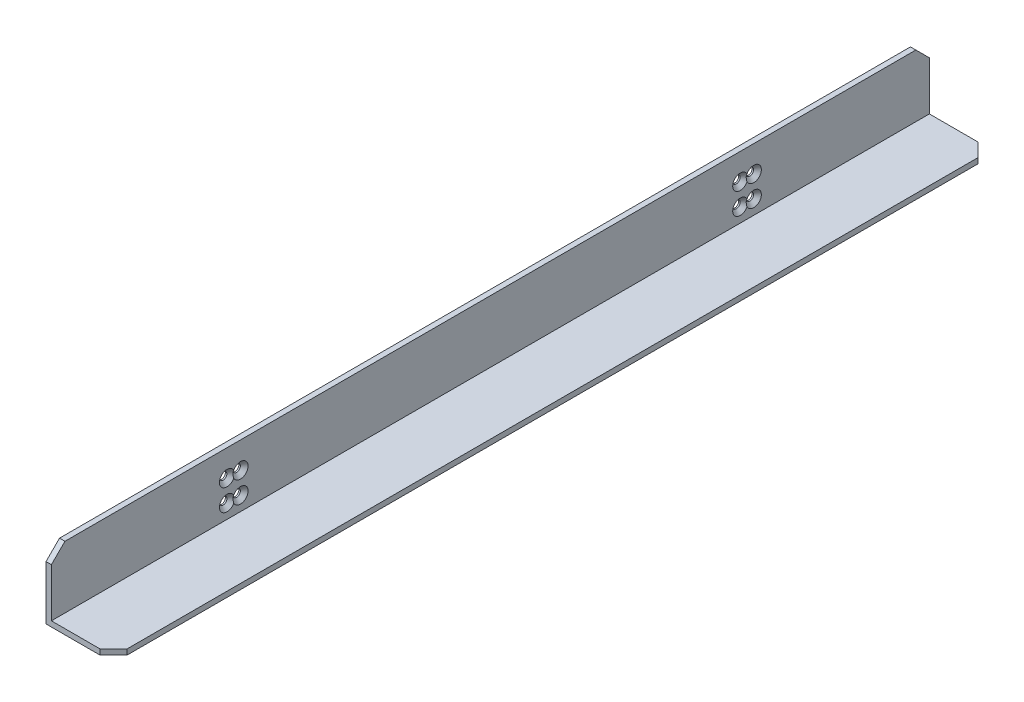
from build123d import *

# Parameters (mm, degrees)
EXTRUDE_1_DEPTH             = 325
CHAMFER_1_SIZE              = 10
HOLE_WIZARD_M5_2_AT_2_COUNT = 2
HOLE_WIZARD_M5_2_AT_2_PITCH = 380
HOLE_WIZARD_M5_2_AT_3_COUNT = 2
HOLE_WIZARD_M5_2_AT_3_PITCH = 10
HOLE_WIZARD_M5_2_AT_4_COUNT = 2
HOLE_WIZARD_M5_2_AT_4_PITCH = 390
HOLE_WIZARD_M5_2_AT_5_COUNT = 2
HOLE_WIZARD_M5_2_AT_5_PITCH = 16
HOLE_WIZARD_M5_2_AT_6_COUNT = 2
HOLE_WIZARD_M5_2_AT_6_PITCH = 380.336692945
HOLE_WIZARD_M5_2_AT_7_COUNT = 2
HOLE_WIZARD_M5_2_AT_7_PITCH = 18.867962264
HOLE_WIZARD_M5_2_AT_8_COUNT = 2
HOLE_WIZARD_M5_2_AT_8_PITCH = 390.328067144


with BuildPart() as part:
    # 草图1 → 凸台-拉伸1 (new, symmetric)
    with BuildSketch(Plane.XY):
        Polygon((0, 0), (50, 0), (50, 4), (4, 4), (4, 50), (0, 50), align=None)
    extrude(amount=EXTRUDE_1_DEPTH, both=True)

    # 倒角1
    chamfer_1_edges = [part.edges().sort_by_distance(p)[0] for p in [
        (50, 2, 325),
        (2, 50, 325),
        (2, 50, -325),
        (50, 2, -325),
    ]]
    chamfer(chamfer_1_edges, length=CHAMFER_1_SIZE)

    # 草图5 → M5 六角凹锥坑螺钉的锥形沉头孔2 (revolve, cut)
    with BuildSketch(Plane(origin=(4, 30.5, 195), x_dir=(0, 0, -1), z_dir=(0, 1, 0))):
        Polygon((0, 0), (0, 4), (2.75, 4), (2.75, 2.85), (5.6, 0), align=None)
    hole_wizard_m5_2 = revolve(axis=Axis((10.35, 30.5, 195), (-1, 0, 0)), mode=Mode.SUBTRACT)

    # M5 六角凹锥坑螺钉的锥形沉头孔2 at 2: M5 六角凹锥坑螺钉的锥形沉头孔2 ×2
    with Locations(*[(0, 0, -i * HOLE_WIZARD_M5_2_AT_2_PITCH) for i in range(1, HOLE_WIZARD_M5_2_AT_2_COUNT)]):
        add(hole_wizard_m5_2, mode=Mode.SUBTRACT)

    # M5 六角凹锥坑螺钉的锥形沉头孔2 at 3: M5 六角凹锥坑螺钉的锥形沉头孔2 ×2
    with Locations(*[(0, 0, -i * HOLE_WIZARD_M5_2_AT_3_PITCH) for i in range(1, HOLE_WIZARD_M5_2_AT_3_COUNT)]):
        add(hole_wizard_m5_2, mode=Mode.SUBTRACT)

    # M5 六角凹锥坑螺钉的锥形沉头孔2 at 4: M5 六角凹锥坑螺钉的锥形沉头孔2 ×2
    with Locations(*[(0, 0, -i * HOLE_WIZARD_M5_2_AT_4_PITCH) for i in range(1, HOLE_WIZARD_M5_2_AT_4_COUNT)]):
        add(hole_wizard_m5_2, mode=Mode.SUBTRACT)

    # M5 六角凹锥坑螺钉的锥形沉头孔2 at 5: M5 六角凹锥坑螺钉的锥形沉头孔2 ×2
    with Locations(*[(0, -i * HOLE_WIZARD_M5_2_AT_5_PITCH, 0) for i in range(1, HOLE_WIZARD_M5_2_AT_5_COUNT)]):
        add(hole_wizard_m5_2, mode=Mode.SUBTRACT)

    # M5 六角凹锥坑螺钉的锥形沉头孔2 at 6: M5 六角凹锥坑螺钉的锥形沉头孔2 ×2
    with Locations(*[Vector(0, -0.04206798948618002, -0.9991147502967769) * (i * HOLE_WIZARD_M5_2_AT_6_PITCH) for i in range(1, HOLE_WIZARD_M5_2_AT_6_COUNT)]):
        add(hole_wizard_m5_2, mode=Mode.SUBTRACT)

    # M5 六角凹锥坑螺钉的锥形沉头孔2 at 7: M5 六角凹锥坑螺钉的锥形沉头孔2 ×2
    with Locations(*[Vector(0, -0.8479983040050839, -0.5299989400031865) * (i * HOLE_WIZARD_M5_2_AT_7_PITCH) for i in range(1, HOLE_WIZARD_M5_2_AT_7_COUNT)]):
        add(hole_wizard_m5_2, mode=Mode.SUBTRACT)

    # M5 六角凹锥坑螺钉的锥形沉头孔2 at 8: M5 六角凹锥坑螺钉的锥形沉头孔2 ×2
    with Locations(*[Vector(0, -0.04099115935241401, -0.9991595092150928) * (i * HOLE_WIZARD_M5_2_AT_8_PITCH) for i in range(1, HOLE_WIZARD_M5_2_AT_8_COUNT)]):
        add(hole_wizard_m5_2, mode=Mode.SUBTRACT)


solid = part.part
